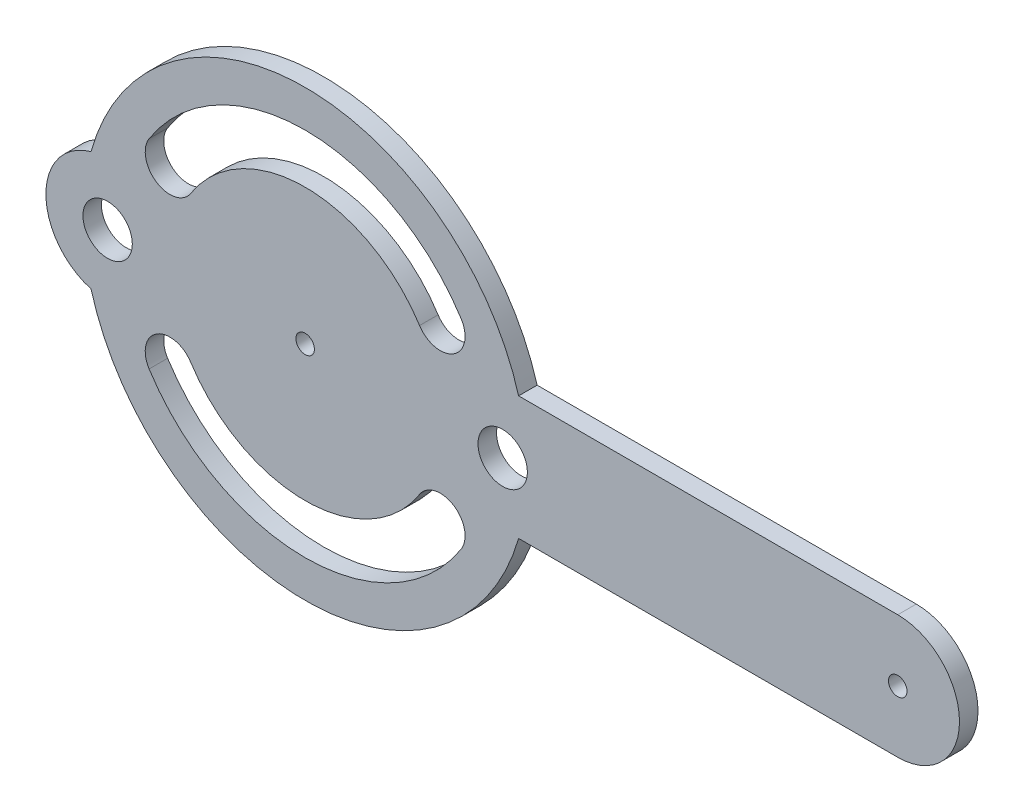
SolidWorks part; units mm, degrees
ref_plane "Front plane" through (0, 0, 0) normal (0, 0, 1) x (1, 0, 0)
ref_plane "Top plane" through (0, 0, 0) normal (0, 1, 0) x (1, 0, 0)
ref_plane "Right plane" through (0, 0, 0) normal (1, 0, 0) x (0, 0, -1)
sketch "Sketch 1" plane through (0, 0, 0) normal (0, 0, 1) x (1, 0, 0)
  line L0 (0, 0) -> (-47.3699, 0) construction
  line L5 (57.6, 0) -> (-16, 0) construction
  line L6 (48, -5) -> (17.2916, -5)
  line L7 (48, 5) -> (17.2916, 5)
  line L8 (0, 0) -> (-10.9543, 7.0002) construction
  line L9 (-10.9543, 7.0002) -> (0, 0) construction
  line L10 (867.9196, 554.631) -> (12.6396, 8.0772) construction
  line L11 (9.269, 5.9232) -> (-10.9543, -7.0002) construction
  arc A15 (-17.3437, -4.816) -> (17.2916, -5) centre (0, 0) ccw
  arc A17 (-17.3437, 4.816) -> (-17.3437, -4.816) centre (-16, 0) ccw
  circle A18 centre (0, 0) radius 0.75
  circle A19 centre (16, 0) radius 2
  circle A20 centre (-16, 0) radius 2
  circle A21 centre (48, 0) radius 0.75
  arc A22 (9.269, 5.9232) -> (-9.269, 5.9232) centre (0, 0) ccw
  arc A24 (9.7509, -8.5976) -> (11.8985, 5.2371) centre (0, 0) ccw construction
  arc A25 (17.2916, 5) -> (-17.3437, 4.816) centre (0, 0) ccw
  arc A26 (-12.6396, 8.0772) -> (-9.269, 5.9232) centre (-10.9543, 7.0002) ccw
  arc A27 (-9.269, -5.9232) -> (-12.6396, -8.0772) centre (-10.9543, -7.0002) ccw
  arc A28 (9.269, 5.9232) -> (12.6396, 8.0772) centre (10.9543, 7.0002) ccw
  arc A29 (12.6396, -8.0772) -> (9.269, -5.9232) centre (10.9543, -7.0002) ccw
  arc A30 (-12.6396, -8.0772) -> (12.6396, -8.0772) centre (0, 0) ccw
  arc A31 (-9.269, -5.9232) -> (9.269, -5.9232) centre (0, 0) ccw
  arc A32 (12.6396, 8.0772) -> (-12.6396, 8.0772) centre (0, 0) ccw
  arc A33 (-10.9543, 7.0002) -> (-10.9543, -7.0002) centre (0, 0) ccw construction
  arc A34 (48, 5) -> (48, -5) centre (48, 0) cw
  point P7 (20.8, 0)
  point P31 (10.9543, 7.0002)
  point P32 (10.9543, -7.0002)
  dimension "D1" = 1.5
  dimension "D2" = 36
  dimension "D3" = 5
  dimension "D4" = 16
  dimension "D6" = 4
  dimension "D9" = 16
  dimension "D8" = 4
  dimension "D10" = 1.5
  dimension "D12" = 22
  dimension "D14" = 26
  dimension "D7" = 16
  dimension "D11" = 48
  dimension "D15" = 32.58
  dimension "D16" = 32.58
extrude "Boss-Extrude 1" add sketch "Sketch 1" along normal blind 1.5
